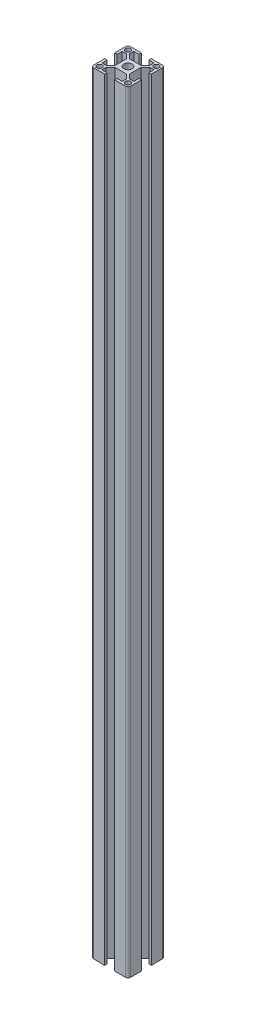
from build123d import *

# Parameters (mm, degrees)
SKETCH_1_R      = 2.1
SKETCH_1_R_2    = 3.4
EXTRUDE_1_DEPTH = 630


with BuildPart() as part:
    # 草图1 → 拉伸1 (new body)
    with BuildSketch(Plane(origin=(0, 0, 0), x_dir=(1, 0, 0), z_dir=(0, 1, 0))):
        with BuildLine():
            Line((6.75, -28), (11, -28))
            Line((11, -28), (11, -30))
            Line((11, -30), (2, -30))
            ThreePointArc((2, -30), (0.585786438, -29.414213562), (0, -28))
            Line((0, -28), (0, -19))
            Line((0, -19), (2, -19))
            Line((2, -19), (2, -23.25))
            Line((2, -23.25), (5.335785999, -23.25))
            Line((5.335785999, -23.25), (9, -19.585785999))
            Line((9, -19.585785999), (9, -10.414214001))
            Line((9, -10.414214001), (5.335785999, -6.75))
            Line((5.335785999, -6.75), (2, -6.75))
            Line((2, -6.75), (2, -11))
            Line((2, -11), (0, -11))
            Line((0, -11), (0, -2))
            ThreePointArc((0, -2), (0.585786438, -0.585786438), (2, 0))
            Line((2, 0), (11, 0))
            Line((11, 0), (11, -2))
            Line((11, -2), (6.75, -2))
            Line((6.75, -2), (6.75, -5.335785999))
            Line((6.75, -5.335785999), (10.414214001, -9))
            Line((10.414214001, -9), (19.585785999, -9))
            Line((19.585785999, -9), (23.25, -5.335785999))
            Line((23.25, -5.335785999), (23.25, -2))
            Line((23.25, -2), (19, -2))
            Line((19, -2), (19, 0))
            Line((19, 0), (28, 0))
            ThreePointArc((28, 0), (29.414213562, -0.585786438), (30, -2))
            Line((30, -2), (30, -11))
            Line((30, -11), (28, -11))
            Line((28, -11), (28, -6.75))
            Line((28, -6.75), (24.664214001, -6.75))
            Line((24.664214001, -6.75), (21, -10.414214001))
            Line((21, -10.414214001), (21, -19.585785999))
            Line((21, -19.585785999), (24.664214001, -23.25))
            Line((24.664214001, -23.25), (28, -23.25))
            Line((28, -23.25), (28, -19))
            Line((28, -19), (30, -19))
            Line((30, -19), (30, -28))
            ThreePointArc((30, -28), (29.414213562, -29.414213562), (28, -30))
            Line((28, -30), (19, -30))
            Line((19, -30), (19, -28))
            Line((19, -28), (23.25, -28))
            Line((23.25, -28), (23.25, -24.664214001))
            Line((23.25, -24.664214001), (19.585785999, -21))
            Line((19.585785999, -21), (10.414214001, -21))
            Line((10.414214001, -21), (6.75, -24.664214001))
            Line((6.75, -24.664214001), (6.75, -28))
        make_face()
        with Locations(Location((3.375, -26.625, 0), (0, 0, 270))):
            Circle(SKETCH_1_R, mode=Mode.SUBTRACT)
        with Locations(Location((26.625, -26.625, 0), (0, 0, 270))):
            Circle(SKETCH_1_R, mode=Mode.SUBTRACT)
        with Locations(Location((15, -15, 0), (0, 0, 270))):
            Circle(SKETCH_1_R_2, mode=Mode.SUBTRACT)
        with Locations(Location((3.375, -3.375, 0), (0, 0, 270))):
            Circle(SKETCH_1_R, mode=Mode.SUBTRACT)
        with Locations(Location((26.625, -3.375, 0), (0, 0, 270))):
            Circle(SKETCH_1_R, mode=Mode.SUBTRACT)
    extrude(amount=EXTRUDE_1_DEPTH)


solid = part.part
